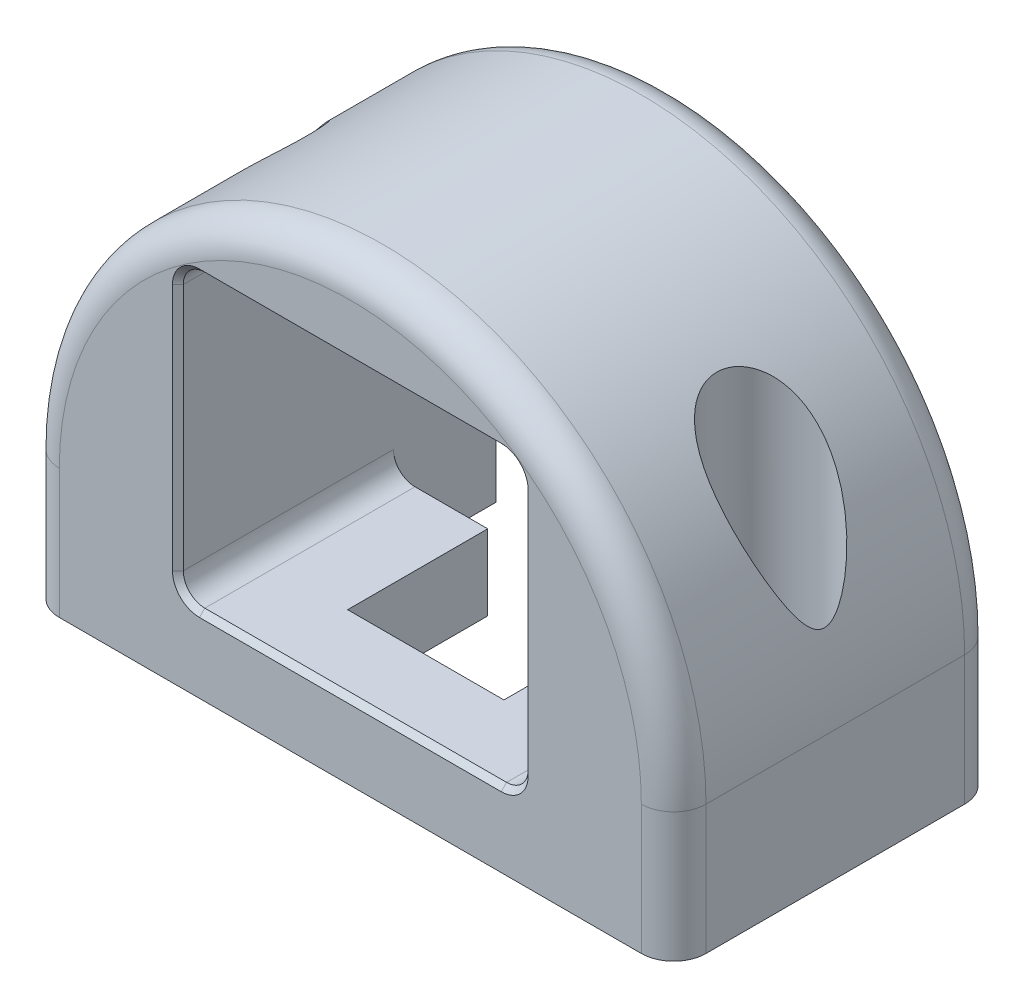
SolidWorks part; units mm, degrees
material "黑賽鋼 "
ref_plane "前基準面" through (0, 0, 0) normal (0, 0, 1) x (1, 0, 0)
ref_plane "上基準面" through (0, 0, 0) normal (0, 1, 0) x (1, 0, 0)
ref_plane "右基準面" through (0, 0, 0) normal (1, 0, 0) x (0, 0, -1)
sketch "草圖1" plane through (0, 0, 0) normal (0, 0, 1) x (1, 0, 0)
  line L0 (55, 0) -> (-55, 0) construction
  line L1 (-30, 0) -> (30, 0)
  line L2 (-30, 0) -> (-30, 12)
  line L4 (30, 0) -> (30, 12)
  line L5 (0, 0) -> (0, 44.0537) construction
  line L6 (0, -55) -> (0, 55) construction
  arc A0 (30, 12) -> (-30, 12) centre (0, 12) ccw
  dimension "D1" = 60
  dimension "D2" = 12
extrude "伸長1" add sketch "草圖1" along normal mid plane 30
ref_plane "平面1" through (0, 50, 0) normal (0, -1, 0) x (1, 0, 0)
hole_wizard "M5 六角承窩頭蓋螺釘的柱孔1" positions "草圖3" profile "草圖2" counterbore size "M5" standard "ISO" end condition through all
sketch "草圖3" plane through (0, 50, 0) normal (0, -1, 0) x (1, 0, 0)
  line L0 (0, 0) -> (0, 38.1441) construction
  line L3 (0, 0) -> (-89.7839, 0) construction
  point P0 (-24, 0)
  point P14 (24, 0)
  dimension "D1" = 48
sketch "草圖2" plane through (-24, 50, 0) normal (1, 0, 0) x (0, 0, 1)
  line L0 (0, 0) -> (0, 50)
  line L1 (0, 50) -> (2.75, 50)
  line L3 (2.75, 50) -> (2.75, 42)
  line L4 (2.75, 42) -> (5, 42)
  line L5 (5, 42) -> (5, 0)
  line L7 (5, 0) -> (0, 0)
  line L11 (0, -6.35) -> (0, 107.95) construction
  dimension "貫穿孔直徑" = 5.5
  dimension "貫穿孔深度" = 50
  dimension "柱孔直徑" = 10
  dimension "柱孔深度" = 42
sketch "草圖4" plane through (0, 0, 15) normal (0, 0, 1) x (1, 0, 0)
  line L0 (0, 0) -> (0, 48.5165) construction
  line L1 (-16, 34) -> (16, 34)
  line L2 (-16, 34) -> (-16, 7)
  line L3 (-16, 7) -> (16, 7)
  line L4 (16, 34) -> (16, 7)
  line L5 (-30, 0) -> (30, 0) construction
  dimension "D1" = 32
  dimension "D2" = 27
  dimension "D3" = 7
extrude "伸長2" cut sketch "草圖4" against normal through all
sketch "草圖5" plane through (0, 7, 0) normal (0, 1, 0) x (1, 0, 0)
  line L0 (-16, 15) -> (-16, 5)
  line L1 (30, 15) -> (-30, 15) construction
  line L2 (-16, 5) -> (-7.25, 5)
  line L3 (-7.25, 5) -> (-7.25, -8)
  line L4 (-7.25, -8) -> (7.25, -8)
  line L5 (0, 0) -> (0, 20.9484) construction
  line L6 (7.25, 5) -> (7.25, -8)
  line L7 (16, 5) -> (7.25, 5)
  line L8 (16, 15) -> (16, 5)
  line L9 (-30, -15) -> (30, -15) construction
  line L10 (-16, 15) -> (16, 15)
  point P11 (0, -8)
  dimension "D1" = 7
  dimension "D2" = 13
  dimension "D3" = 14.5
  dimension "D4" = 32
extrude "伸長3" cut sketch "草圖5" against normal through all
fillet "圓角1" radius 2 4 edges at (16, 7, 5) (-16, 7, 5) (-16, 34, 0) (16, 34, 0)
fillet "圓角2" radius 3 6 edges at (30, 6, 15) (-30, 6, 15) (30, 6, -15) (-30, 6, -15) (0, 42, 15) (0, 42, -15)
chamfer "導角1" distance 0.5 angle 45 13 edges at (0, 34, 15) (-15.4142, 33.4142, 15) (15.4142, 33.4142, 15) (-16, 20.5, 15) (16, 20.5, 15) (-15.4142, 7.5858, 15) (15.4142, 7.5858, 15) (0, 7, 15) (16, 16, -15) (15.4142, 33.4142, -15) (0, 34, -15) (-15.4142, 33.4142, -15) (-16, 16, -15)
